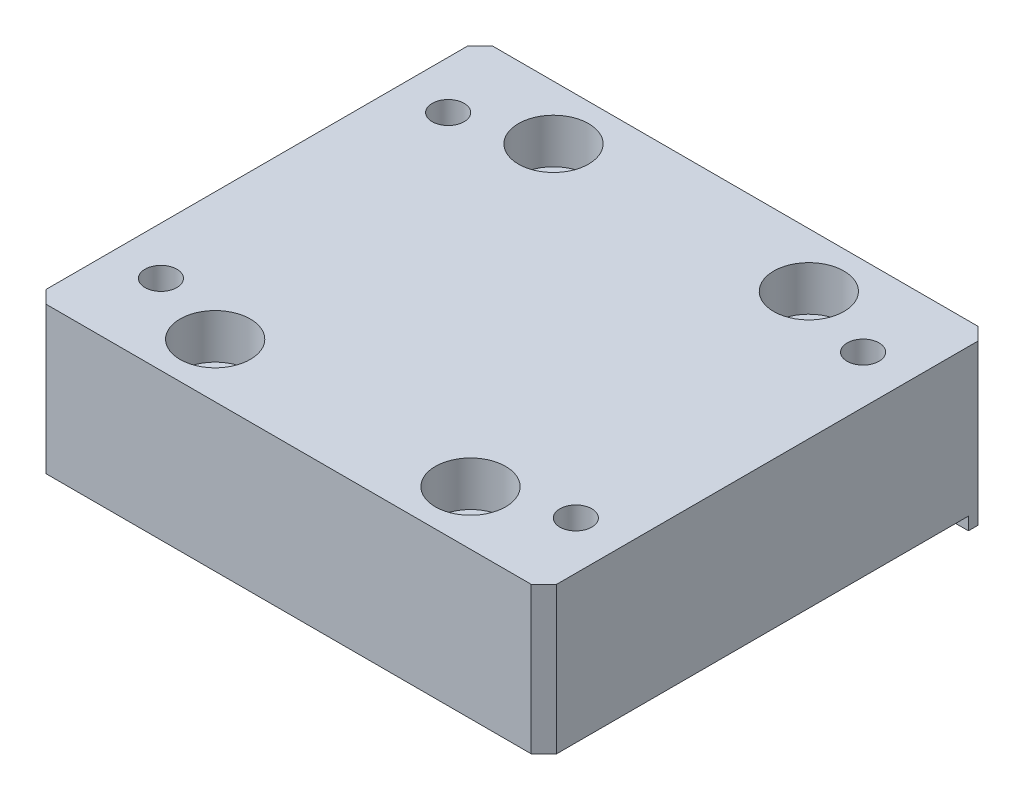
SolidWorks part; units mm, degrees
material "6061"
ref_plane "前视基准面" through (0, 0, 0) normal (0, 0, 1) x (1, 0, 0)
ref_plane "上视基准面" through (0, 0, 0) normal (0, 1, 0) x (1, 0, 0)
ref_plane "右视基准面" through (0, 0, 0) normal (1, 0, 0) x (0, 0, -1)
sketch "草图1" plane through (0, 0, 0) normal (0, 1, 0) x (1, 0, 0)
  line L1 (40, -35) -> (-40, -35)
  line L2 (40, -35) -> (40, 35)
  line L3 (40, 35) -> (-40, 35)
  line L4 (-40, -35) -> (-40, 35)
  line L5 (40, -35) -> (-40, 35) construction
  line L6 (40, 35) -> (-40, -35) construction
  point P0 (0, 0)
  dimension "D1" = 80
  dimension "D2" = 70
extrude "凸台-拉伸1" add sketch "草图1" along normal mid plane 25
sketch "草图3" plane through (0, -12.5, 0) normal (0, -1, 0) x (1, 0, 0)
  line L0 (-40, -35) -> (-40, 35) construction
  line L1 (40, 35) -> (-40, 35)
  line L2 (40, 35) -> (40, -31.5)
  line L3 (40, -31.5) -> (-40, -31.5)
  line L4 (-40, 35) -> (-40, -31.5)
  line L5 (40, -35) -> (-40, -35) construction
  dimension "D1" = 3.5
extrude "切除-拉伸1" cut sketch "草图3" against normal blind 2
hole_wizard "M5 螺纹孔1" positions "草图4" profile "草图5" tap size "M5" standard "ISO" end condition through all
sketch "草图4" plane through (0, -10.5, 0) normal (0, -1, 0) x (-1, 0, 0)
  point P0 (20, 26.5)
  point P3 (-20, 26.5)
  point P6 (-20, -26.5)
  point P9 (20, -26.5)
sketch "草图5" plane through (-20, -10.5, -26.5) normal (1, 0, 0) x (0, 0, -1)
  line L0 (0, 0) -> (0, 23)
  line L1 (0, 23) -> (2.1, 23)
  line L2 (2.1, 23) -> (2.1, 0)
  line L5 (2.1, 0) -> (0, 0)
  line L11 (0, -6.35) -> (0, 107.95) construction
  dimension "通孔螺纹孔钻头直径" = 4.2
  dimension "通孔螺纹孔钻头深度" = 23
cosmetic thread "孔螺蚊线1" parameters "D1"=13, "D2"=5
cosmetic thread "孔螺蚊线2" parameters "D1"=13, "D2"=5
cosmetic thread "孔螺蚊线3" parameters "D1"=13, "D2"=5
cosmetic thread "孔螺蚊线4" parameters "D1"=13, "D2"=5
hole_wizard "M6 螺纹孔1" positions "草图6" profile "草图7" tap size "M6" standard "ISO" end condition through all
sketch "草图6" plane through (0, -10.5, 0) normal (0, -1, 0) x (-1, 0, 0)
  line L1 (32.5, 22.5) -> (-32.5, 22.5)
  line L2 (32.5, 22.5) -> (32.5, -22.5)
  line L3 (32.5, -22.5) -> (-32.5, -22.5)
  line L4 (-32.5, 22.5) -> (-32.5, -22.5)
  line L5 (32.5, 22.5) -> (-32.5, -22.5)
  point P0 (32.5, 22.5)
  point P2 (32.5, -22.5)
  point P4 (-32.5, 22.5)
  point P6 (-32.5, -22.5)
  dimension "D1" = 45
  dimension "D2" = 65
sketch "草图7" plane through (-32.5, -10.5, -22.5) normal (1, 0, 0) x (0, 0, -1)
  line L0 (0, 0) -> (0, 23)
  line L1 (0, 23) -> (2.5, 23)
  line L2 (2.5, 23) -> (2.5, 0)
  line L5 (2.5, 0) -> (0, 0)
  line L11 (0, -6.35) -> (0, 107.95) construction
  dimension "通孔螺纹孔钻头直径" = 5
  dimension "通孔螺纹孔钻头深度" = 23
cosmetic thread "孔螺蚊线5" parameters "D2"=6
cosmetic thread "孔螺蚊线6" parameters "D2"=6
cosmetic thread "孔螺蚊线7" parameters "D2"=6
cosmetic thread "孔螺蚊线8" parameters "D2"=6
chamfer "倒角1" distance 2 angle 45 4 edges at (-40, 1, 35) (40, 1, 35) (40, 0, -35) (-40, 0, -35)
hole_wizard "打孔尺寸(%根据)内六角花形圆柱头螺钉1" positions "草图8" profile "草图9" counterbore size "M6" standard "GB" end condition up to next
sketch "草图8" plane through (0, 12.5, 0) normal (0, 1, 0) x (1, 0, 0)
  point P0 (20, 26.5)
  point P3 (20, -26.5)
  point P6 (-20, -26.5)
  point P9 (-20, 26.5)
sketch "草图9" plane through (20, 12.5, -26.5) normal (1, 0, 0) x (0, 0, 1)
  line L0 (0, 0) -> (0, 25)
  line L1 (0, 25) -> (3.3, 25)
  line L3 (3.3, 25) -> (3.3, 7)
  line L4 (3.3, 7) -> (5.5, 7)
  line L5 (5.5, 7) -> (5.5, 0)
  line L7 (5.5, 0) -> (0, 0)
  line L11 (0, -6.35) -> (0, 107.95) construction
  dimension "通孔孔直径" = 6.6
  dimension "通孔孔深度" = 25
  dimension "柱形沉头孔直径" = 11
  dimension "柱形沉头孔深度" = 7
